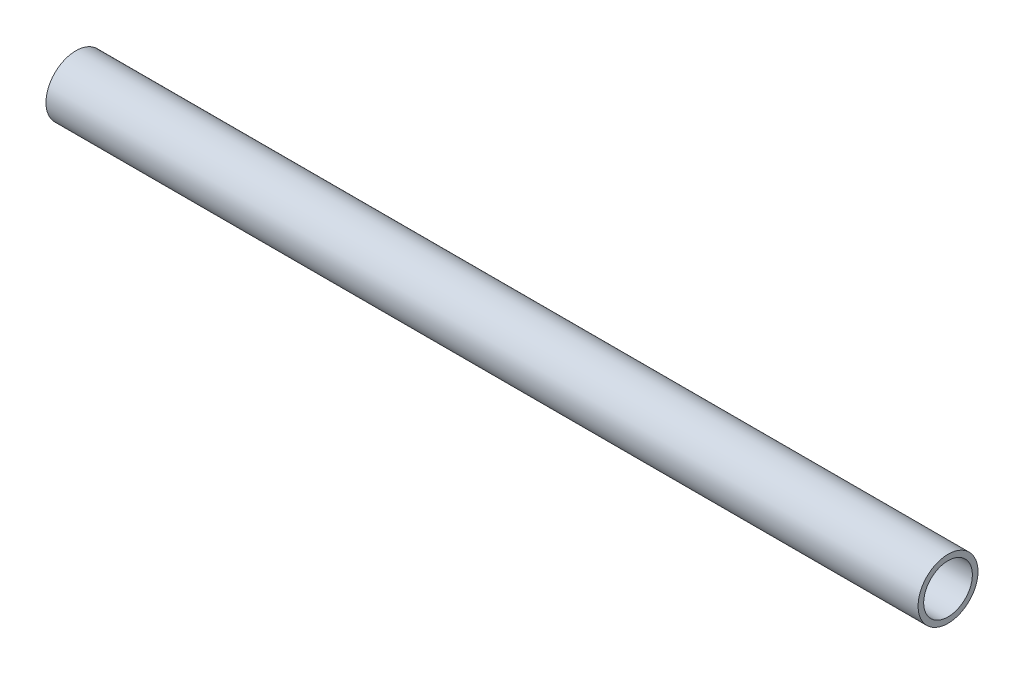
from build123d import *

# Parameters (mm, degrees)
SKETCH1_R                                  = 10.65
SKETCH1_R_2                                = 8.65
GB_T6728_2002_ROUND_TUBE_021_3_X_2_1_DEPTH = 310


with BuildPart() as part:
    # Sketch1 → Gb／t6728-2002 round tube 021.3 X 2 (1) (new body)
    with BuildSketch(Plane(origin=(-155, 0, 0), x_dir=(0, 0, -1), z_dir=(1, 0, 0))):
        Circle(SKETCH1_R)
        Circle(SKETCH1_R_2, mode=Mode.SUBTRACT)
    extrude(amount=GB_T6728_2002_ROUND_TUBE_021_3_X_2_1_DEPTH)


solid = part.part
